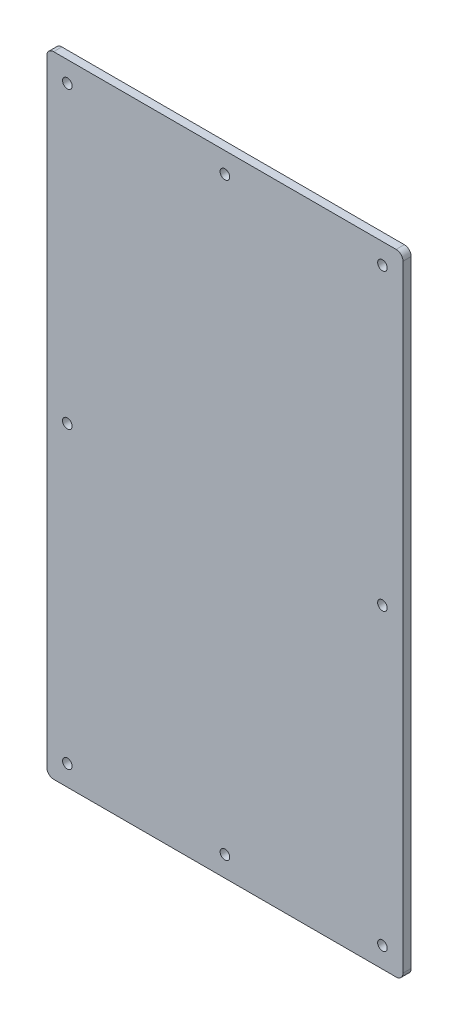
SolidWorks part; units mm, degrees
ref_plane "前视" through (0, 0, 0) normal (0, 0, 1) x (1, 0, 0)
ref_plane "上视" through (0, 0, 0) normal (0, 1, 0) x (1, 0, 0)
ref_plane "右视" through (0, 0, 0) normal (1, 0, 0) x (0, 0, -1)
sketch "草图1" plane through (0, 0, 0) normal (0, 0, 1) x (1, 0, 0)
  line L1 (0, 0) -> (260, 0)
  line L2 (0, 0) -> (0, -460)
  line L3 (0, -460) -> (260, -460)
  line L4 (260, 0) -> (260, -460)
  dimension "D1" = 260
  dimension "D2" = 460
extrude "凸台-拉伸1" add sketch "草图1" along normal blind 6
fillet "圆角1" radius 5 4 edges at (0, -460, 3) (260, -460, 3) (260, 0, 3) (0, 0, 3)
sketch "草图2" plane through (0, 0, 0) normal (0, 0, -1) x (-1, 0, 0)
  line L0 (-130, -460) -> (-130, 0) construction
  line L1 (-5, -460) -> (-255, -460) construction
  line L2 (-255, 0) -> (-5, 0) construction
  line L3 (0, -5) -> (0, -455) construction
  line L4 (-15, -445) -> (-245, -445) construction
  line L5 (-15, -445) -> (-15, -15) construction
  line L6 (-15, -15) -> (-245, -15) construction
  line L7 (-245, -445) -> (-245, -15) construction
  line L8 (-15, -445) -> (-245, -15) construction
  line L9 (-15, -15) -> (-245, -445) construction
  circle A0 centre (-245, -445) radius 3.5
  circle A1 centre (-15, -445) radius 3.5
  circle A2 centre (-245, -15) radius 3.5
  circle A3 centre (-15, -15) radius 3.5
  circle A4 centre (-130, -445) radius 3.5
  circle A5 centre (-245, -230) radius 3.5
  circle A6 centre (-130, -15) radius 3.5
  circle A7 centre (-15, -230) radius 3.5
  point P6 (-130, -230)
  dimension "D3" = 7
  dimension "D1" = 15
  dimension "D2" = 15
extrude "切除-拉伸1" cut sketch "草图2" against normal through all
